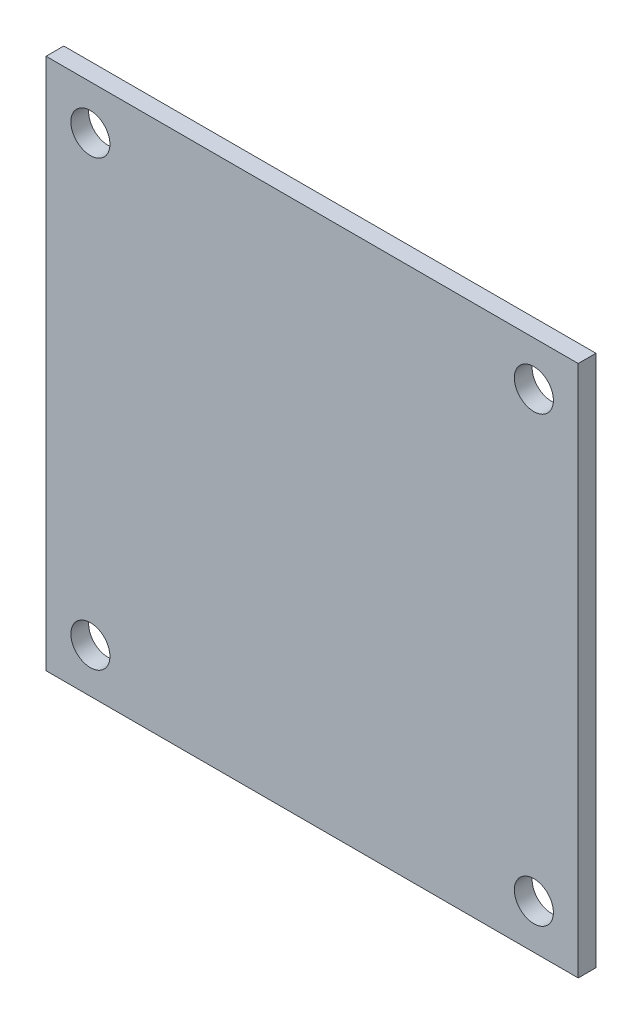
SolidWorks part; units mm, degrees
ref_plane "Front Plane" through (0, 0, 0) normal (0, 0, 1) x (1, 0, 0)
ref_plane "Top Plane" through (0, 0, 0) normal (0, 1, 0) x (1, 0, 0)
ref_plane "Right Plane" through (0, 0, 0) normal (1, 0, 0) x (0, 0, -1)
other "Configuration Table"
sketch "Sketch1" plane through (0, 0, 0) normal (0, 0, 1) x (1, 0, 0)
  line L1 (-150, 150) -> (150, 150)
  line L2 (-150, 150) -> (-150, -150)
  line L3 (-150, -150) -> (150, -150)
  line L4 (150, 150) -> (150, -150)
  line L5 (-150, 150) -> (150, -150) construction
  line L6 (-150, -150) -> (150, 150) construction
  line L7 (-125, 125) -> (125, 125) construction
  line L8 (-125, 125) -> (-125, -125) construction
  line L9 (-125, -125) -> (125, -125) construction
  line L10 (125, 125) -> (125, -125) construction
  line L11 (-125, 125) -> (125, -125) construction
  line L12 (-125, -125) -> (125, 125) construction
  circle A0 centre (-125, 125) radius 11
  circle A1 centre (125, 125) radius 11
  circle A2 centre (125, -125) radius 11
  circle A3 centre (-125, -125) radius 11
  point P0 (0, 0)
  point P6 (0, 0)
  dimension "D4" = 22
  dimension "D1" = 300
  dimension "D2" = 250
  dimension "400" = 300
  dimension "D3" = 250
extrude "Boss-Extrude1" add sketch "Sketch1" along normal blind 10
